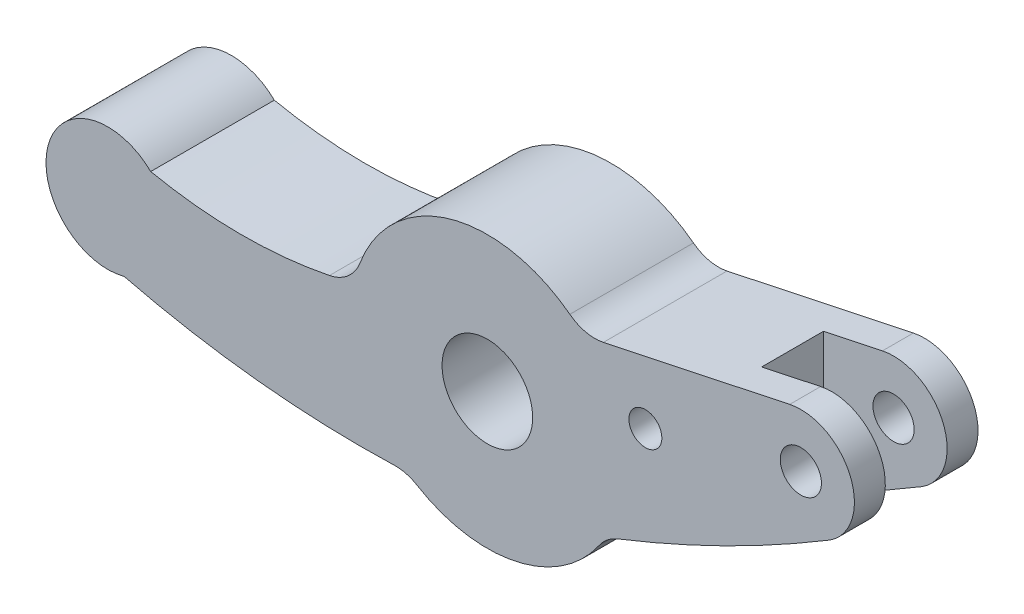
SolidWorks part; units mm, degrees
ref_plane "Front Plane" through (0, 0, 0) normal (0, 0, 1) x (1, 0, 0)
ref_plane "Top Plane" through (0, 0, 0) normal (0, 1, 0) x (1, 0, 0)
ref_plane "Right Plane" through (0, 0, 0) normal (1, 0, 0) x (0, 0, -1)
sketch "Sketch1" plane through (0, 0, 0) normal (0, 0, 1) x (1, 0, 0)
  line L7 (23.3648, -2.4326) -> (82.7627, 3.0066)
  line L8 (23.3729, -8.3627) -> (82.7596, -3.0293)
  arc A14 (23.3648, -2.4326) -> (23.3729, -8.3627) centre (8.6648, -5.4177) ccw
  arc A16 (82.7596, -3.0293) -> (82.7627, 3.0066) centre (100.5064, -0.0205) ccw
extrude "Boss-Extrude1" add sketch "Sketch1" along normal blind 10
sketch "Sketch7" plane through (0, 0, 0) normal (0, 0, -1) x (-1, 0, 0)
  circle A0 centre (-100.78, 0) radius 8
extrude "Cut-Extrude2" cut sketch "Sketch7" against normal blind 10
sketch "Sketch8" plane through (0, 0, 10) normal (0, 0, 1) x (1, 0, 0)
  circle A0 centre (8.6648, -5.4177) radius 6
extrude "Cut-Extrude3" cut sketch "Sketch8" against normal blind 14
sketch "Sketch17" plane through (0, 0, 0) normal (0, 0, -1) x (-1, 0, 0)
  line L1 (-115.8122, 9.3934) -> (-161.8976, 22.2751)
  line L2 (-118.4017, 1.9179) -> (-164.5896, 12.6443)
  arc A0 (-161.8976, 22.2751) -> (-164.5896, 12.6443) centre (-176.8637, 21.2668) ccw
  arc A1 (-118.4017, 1.9179) -> (-115.8122, 9.3934) centre (-100.78, 0) ccw
  circle A2 centre (-100.78, 0) radius 8
  arc A3 (-82.7627, 3.0066) -> (-82.7596, -3.0293) centre (-100.5064, -0.0205) ccw construction
  point P4 (-99.434, 4.8154)
  point P5 (-175.5177, 26.0822)
  point P6 (-102.126, -4.8154)
  point P7 (-178.2097, 16.4513)
extrude "Boss-Extrude2" add sketch "Sketch17" against normal blind 10
sketch "Sketch18" plane through (0, 0, 0) normal (0, 0, -1) x (-1, 0, 0)
  circle A0 centre (-176.8637, 21.2668) radius 6
extrude "Cut-Extrude10" cut sketch "Sketch18" against normal blind 10
sketch "Sketch20" plane through (0, 0, 10) normal (0, 0, 1) x (1, 0, 0)
  circle A0 centre (176.8637, 21.2668) radius 15
sketch "Sketch21" plane through (0, 0, 10) normal (0, 0, 1) x (1, 0, 0)
  circle A0 centre (8.6648, -5.4177) radius 15
sketch "Sketch22" plane through (0, 0, 10) normal (0, 0, 1) x (1, 0, 0)
  circle A0 centre (8.6648, -5.4177) radius 13
sketch "Sketch23" plane through (0, 0, 10) normal (0, 0, 1) x (1, 0, 0)
  line L0 (174.169, 33.9844) -> (97.0897, 17.6522)
  line L1 (181.1377, 8.9894) -> (108.1783, -16.4093)
  arc A0 (8.6648, -18.4177) -> (102.3485, -17.9315) centre (54.4178, 191.6593) ccw
  arc A3 (13.0493, 6.8206) -> (92.6784, 16.1882) centre (41.1609, 110.9854) ccw
  arc A6 (181.1377, 8.9894) -> (174.169, 33.9844) centre (176.8637, 21.2668) ccw
  arc A10 (13.0493, 6.8206) -> (8.6648, -18.4177) centre (8.6648, -5.4177) ccw
  arc A11 (102.3485, -17.9315) -> (108.1783, -16.4093) centre (100.78, 0) ccw
  arc A12 (92.6784, 16.1882) -> (97.0897, 17.6522) centre (100.5064, -0.0205) cw
extrude "Boss-Extrude3" add sketch "Sketch23" along normal blind 10
sketch "Sketch25" plane through (0, 0, 10) normal (0, 0, -1) x (-1, 0, 0)
  circle A0 centre (-8.6648, -5.4177) radius 5
extrude "Cut-Extrude11" cut sketch "Sketch25" against normal blind 20
sketch "Sketch26" plane through (0, 0, 20) normal (0, 0, 1) x (1, 0, 0)
  circle A0 centre (8.6648, -5.4177) radius 8.5
sketch "Sketch29" plane through (0, 0, 10) normal (0, 0, -1) x (-1, 0, 0)
  circle A0 centre (-176.8637, 21.2668) radius 5
extrude "Cut-Extrude12" cut sketch "Sketch29" against normal blind 10
sketch "Sketch30" plane through (0, 0, 0) normal (0, 0, -1) x (-1, 0, 0)
  line L2 (-181.1377, 8.9894) -> (-108.1783, -16.4093)
  line L3 (-97.0897, 17.6522) -> (-174.169, 33.9844)
  line L4 (-181.1377, 8.9894) -> (-108.1783, -16.4093)
  line L5 (-97.0897, 17.6522) -> (-174.169, 33.9844)
  arc A6 (-8.6648, -18.4177) -> (-13.0493, 6.8206) centre (-8.6648, -5.4177) ccw
  arc A7 (-102.3485, -17.9315) -> (-8.6648, -18.4177) centre (-54.4178, 191.6593) ccw
  arc A8 (-108.1783, -16.4093) -> (-102.3485, -17.9315) centre (-100.78, 0) ccw
  arc A9 (-174.169, 33.9844) -> (-181.1377, 8.9894) centre (-176.8637, 21.2668) ccw
  arc A10 (-92.6784, 16.1882) -> (-97.0897, 17.6522) centre (-100.5064, -0.0205) ccw
  arc A11 (-92.6784, 16.1882) -> (-13.0493, 6.8206) centre (-41.1609, 110.9854) ccw
  arc A12 (-8.6648, -18.4177) -> (-13.0493, 6.8206) centre (-8.6648, -5.4177) ccw
  arc A13 (-102.3485, -17.9315) -> (-8.6648, -18.4177) centre (-54.4178, 191.6593) ccw
  arc A14 (-108.1783, -16.4093) -> (-102.3485, -17.9315) centre (-100.78, 0) ccw
  arc A15 (-174.169, 33.9844) -> (-181.1377, 8.9894) centre (-176.8637, 21.2668) ccw
  arc A16 (-92.6784, 16.1882) -> (-97.0897, 17.6522) centre (-100.5064, -0.0205) ccw
  arc A17 (-92.6784, 16.1882) -> (-13.0493, 6.8206) centre (-41.1609, 110.9854) ccw
  dimension "D1" = 0
sketch "Sketch31" plane through (0, 0, 10) normal (0, 0, -1) x (-1, 0, 0)
  circle A0 centre (-100.78, 0) radius 11
extrude "Cut-Extrude13" cut sketch "Sketch31" against normal blind 10
extrude "Boss-Extrude5" add sketch "Sketch30" along normal blind 10 and the other way blind 10 contours L5 A15 L4 A14 A13 A12 A17 A16
sketch "Sketch32" plane through (0, 0, 10) normal (0, 0, 1) x (1, 0, 0)
  circle A0 centre (8.6648, -5.4177) radius 5
  circle A1 centre (100.78, 0) radius 11
  circle A2 centre (176.8637, 21.2668) radius 5
extrude "Cut-Extrude14" cut sketch "Sketch32" against normal blind 20
ref_plane "Plane1" through (0, 0, -2.5) normal (0, 0, -1) x (-1, 0, 0)
sketch "Sketch33" plane through (0, 0, -2.5) normal (0, 0, -1) x (-1, 0, 0)
  line L1 (-25.6648, -5.4177) -> (-25.6648, -33.5873)
  line L2 (-25.6648, -33.5873) -> (16.718, -33.5873)
  line L3 (16.718, -33.5873) -> (16.718, 17.6907)
  line L4 (16.718, 17.6907) -> (-25.6648, 17.6907)
  line L5 (-25.6648, 17.6907) -> (-25.6648, -5.4177)
  line L6 (-159.8637, -3.5732) -> (-159.8637, 44.7912)
  line L7 (-159.8637, -3.5732) -> (-203.6907, -3.5732)
  line L8 (-203.6907, -3.5732) -> (-203.6907, 44.7912)
  line L9 (-203.6907, 44.7912) -> (-159.8637, 44.7912)
extrude "Cut-Extrude15" cut sketch "Sketch33" against normal blind 15
sketch "Sketch36" plane through (0, 0, 20) normal (0, 0, 1) x (1, 0, 0)
  circle A0 centre (139.1279, 11.3772) radius 4
sketch "Sketch37" plane through (0, 0, 20) normal (0, 0, 1) x (1, 0, 0)
  circle A0 centre (8.6648, -5.4177) radius 15
sketch "Sketch38" plane through (0, 0, -10) normal (0, 0, -1) x (-1, 0, 0)
  line L3 (-183.9213, 10.3494) -> (-165.5775, 5.1601)
  line L4 (-165.5775, 5.1601) -> (-95.9299, -17.1103)
  line L5 (-95.9299, -17.1103) -> (-5.6959, -18.0741)
  arc A0 (-111.0892, -22.7754) -> (-100.78, -25) centre (-100.78, 0) ccw
  arc A3 (-174.169, 33.9844) -> (-181.1377, 8.9894) centre (-176.8637, 21.2668) ccw construction
  arc A5 (-5.6959, -18.0741) -> (-100.78, -25) centre (-70.4038, 214.1305) cw
  arc A6 (-183.9213, 10.3494) -> (-111.0892, -22.7754) centre (-6.8528, 303.0422) ccw
extrude "Boss-Extrude7" add sketch "Sketch38" against normal up to surface (30 mm away)
sketch "Sketch39" plane through (0, 0, 0) normal (0, 1, 0) x (1, 0, 0)
  line L0 (-4.3352, 2.5) -> (25.6648, 2.5)
  line L1 (25.6648, 2.5) -> (25.6648, -12.5)
  line L2 (25.6648, -12.5) -> (-5.8603, -12.5)
  line L3 (-5.8603, -12.5) -> (-4.3352, 2.5)
  line L4 (159.8637, 2.5) -> (191.0122, 2.5)
  line L5 (191.0122, 2.5) -> (191.0122, -12.5)
  line L6 (191.0122, -12.5) -> (159.8637, -12.5)
  line L7 (159.8637, -12.5) -> (159.8637, 2.5)
extrude "Cut-Extrude16" cut sketch "Sketch39" against normal blind 62 and the other way blind 66
extrude "Cut-Extrude17" cut sketch "Sketch36" against normal blind 15
sketch "Sketch40" plane through (0, 0, 20) normal (0, 0, 1) x (1, 0, 0)
  circle A0 centre (100.78, 0) radius 33
  circle A1 centre (100.78, 0) radius 11
extrude "Boss-Extrude8" add sketch "Sketch40" against normal up to surface (30 mm away) up to face at (108.9663, 5.3915, -10)
fillet "Fillet1" radius 10 4 edges at (124.0782, 23.3708, 5) (68.447, 6.6013, 5) (129.4653, -16.3142, 5) (81.3493, -26.673, 5)
ref_plane "Plane2" through (0, 0, 18.5) normal (0, 0, 1) x (1, 0, 0)
ref_plane "Plane3" through (0, 0, -8.5) normal (0, 0, -1) x (-1, 0, 0)
ref_plane "Plane4" through (0, 0, 5) normal (0, 0, -1) x (-1, 0, 0)
sketch "Sketch47" plane through (0, 0, 20) normal (0, 0, 1) x (1, 0, 0)
  line L0 (62.4634, 5.2179) -> (78.1975, -26.7956)
  arc A0 (19.0791, 5.3779) -> (12.6076, -19.8902) centre (8.6648, -5.4177) ccw
  arc A1 (5.6959, -18.0741) -> (78.1975, -26.7956) centre (70.4038, 214.1305) ccw construction
  arc A2 (13.0493, 6.8206) -> (62.4634, 5.2179) centre (41.1609, 110.9854) ccw construction
  arc A3 (12.6076, -19.8902) -> (78.1975, -26.7956) centre (70.4038, 214.1305) ccw
  arc A4 (19.0791, 5.3779) -> (62.4634, 5.2179) centre (41.1609, 110.9854) ccw
  dimension "D1" = 30
extrude "Boss-Extrude10" add sketch "Sketch47" against normal up to surface (30 mm away) up to face at (105.4088, 3.6334, -10)
